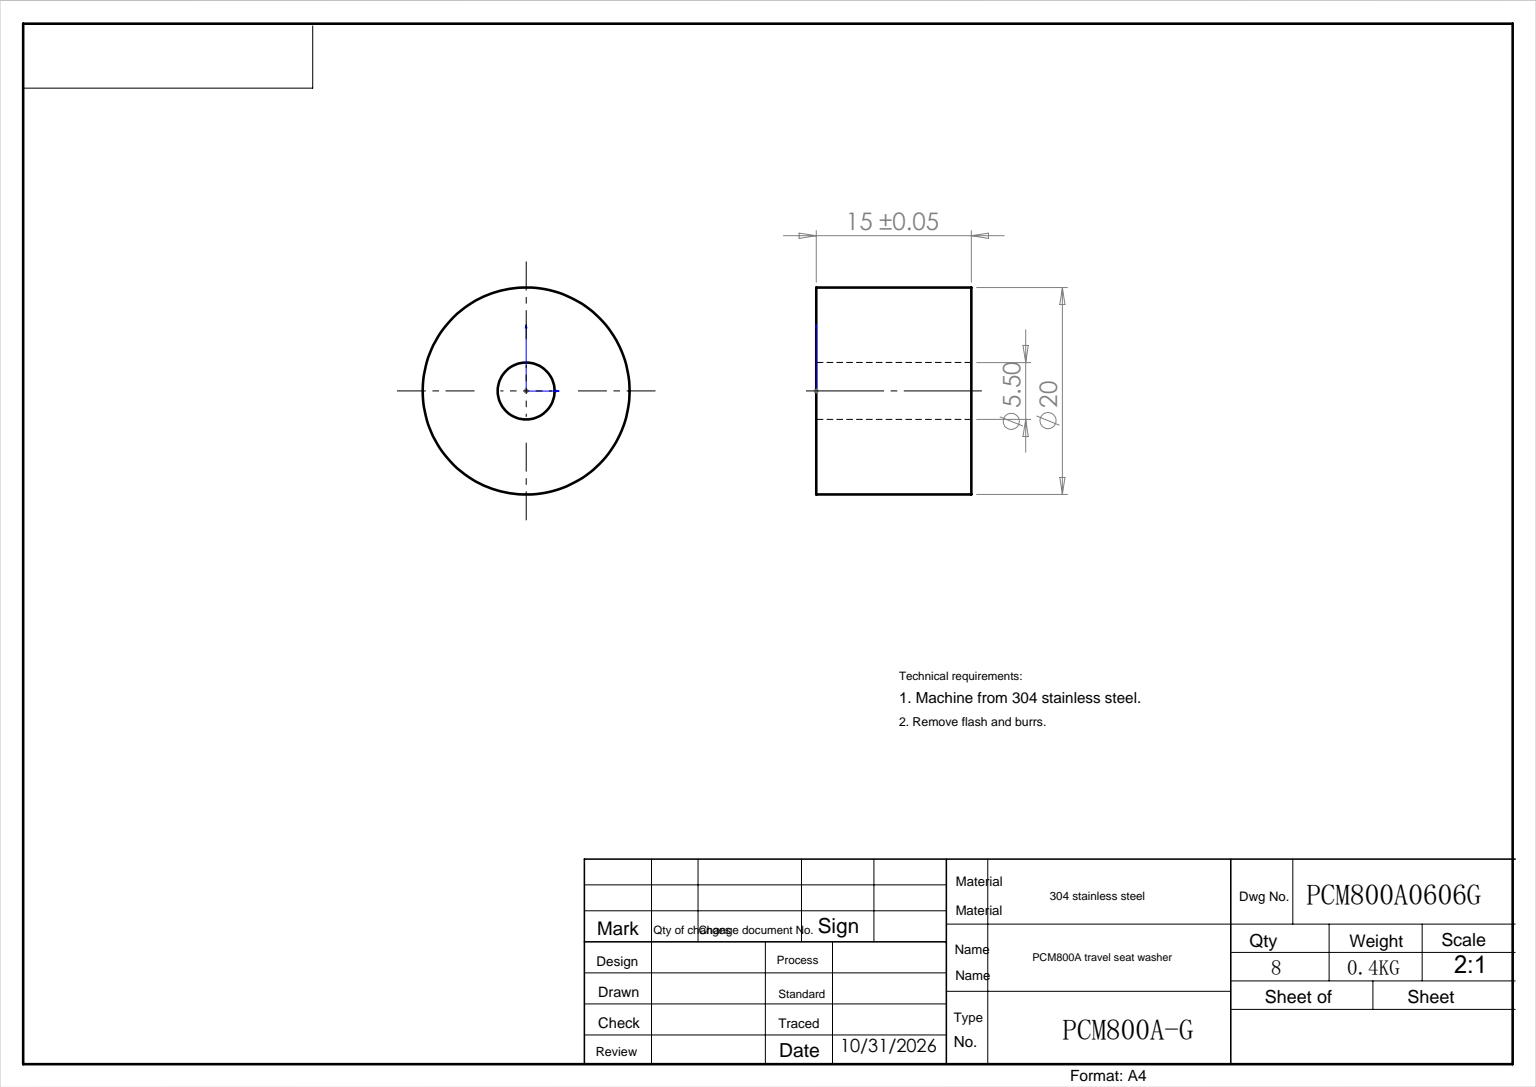
SolidWorks part; units mm, degrees
ref_plane "前视基准面" through (0, 0, 0) normal (0, 0, 1) x (1, 0, 0)
ref_plane "上视基准面" through (0, 0, 0) normal (0, 1, 0) x (1, 0, 0)
ref_plane "右视基准面" through (0, 0, 0) normal (1, 0, 0) x (0, 0, -1)
sketch "草图1" plane through (0, 0, 0) normal (0, 0, 1) x (1, 0, 0)
  circle A0 centre (0, 0) radius 10
  circle A1 centre (0, 0) radius 2.75
  dimension "D1" = 20
  dimension "D2" = 5.5
extrude "凸台-拉伸1" add sketch "草图1" along normal blind 15
